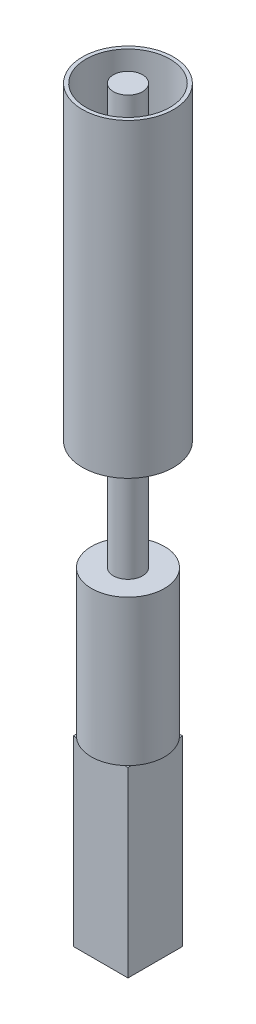
from build123d import *

# Parameters (mm, degrees)
SKETCH1_R           = 8
BOSS_EXTRUDE1_DEPTH = 230
SKETCH3_R           = 25
SKETCH3_R_2         = 23
BOSS_EXTRUDE2_DEPTH = 170
BOSS_EXTRUDE3_START = 80
SKETCH4_W           = 30
SKETCH4_H           = 30
BOSS_EXTRUDE3_DEPTH = 100
SKETCH5_R           = 20
BOSS_EXTRUDE4_DEPTH = 80


with BuildPart() as part:
    # Sketch1 → Boss-Extrude1 (new body)
    with BuildSketch(Plane(origin=(0, 0, 0), x_dir=(1, 0, 0), z_dir=(0, 1, 0))):
        with Locations(Location((0, 0, 0), (0, 0, 270))):
            Circle(SKETCH1_R)
    extrude(amount=BOSS_EXTRUDE1_DEPTH)



with BuildPart() as body_2:
    # Sketch3 → Boss-Extrude2 (new body)
    with BuildSketch(Plane(origin=(0, 230, 0), x_dir=(1, 0, 0), z_dir=(0, 1, 0))):
        with Locations(Location((0, 0, 0), (0, 0, 270))):
            Circle(SKETCH3_R)
        with Locations(Location((0, 0, 0), (0, 0, 270))):
            Circle(SKETCH3_R_2, mode=Mode.SUBTRACT)
    extrude(amount=-BOSS_EXTRUDE2_DEPTH)


with BuildPart() as body_3:
    # Sketch4 → Boss-Extrude3 (new body)
    with BuildSketch(Plane.XZ.offset(BOSS_EXTRUDE3_START)):
        Rectangle(SKETCH4_W, SKETCH4_H)
    extrude(amount=BOSS_EXTRUDE3_DEPTH)


with BuildPart() as part_1:
    add(part.part)

    add(body_3.part)  # Boss-Extrude4 merges body 3
    # Sketch5 → Boss-Extrude4 (add)
    with BuildSketch(Plane.XZ):
        with Locations(Location((0, 0, 0), (0, 0, 131.409622109))):
            Circle(SKETCH5_R)
    extrude(amount=BOSS_EXTRUDE4_DEPTH)


solid = Compound([body_2.part, part_1.part])
